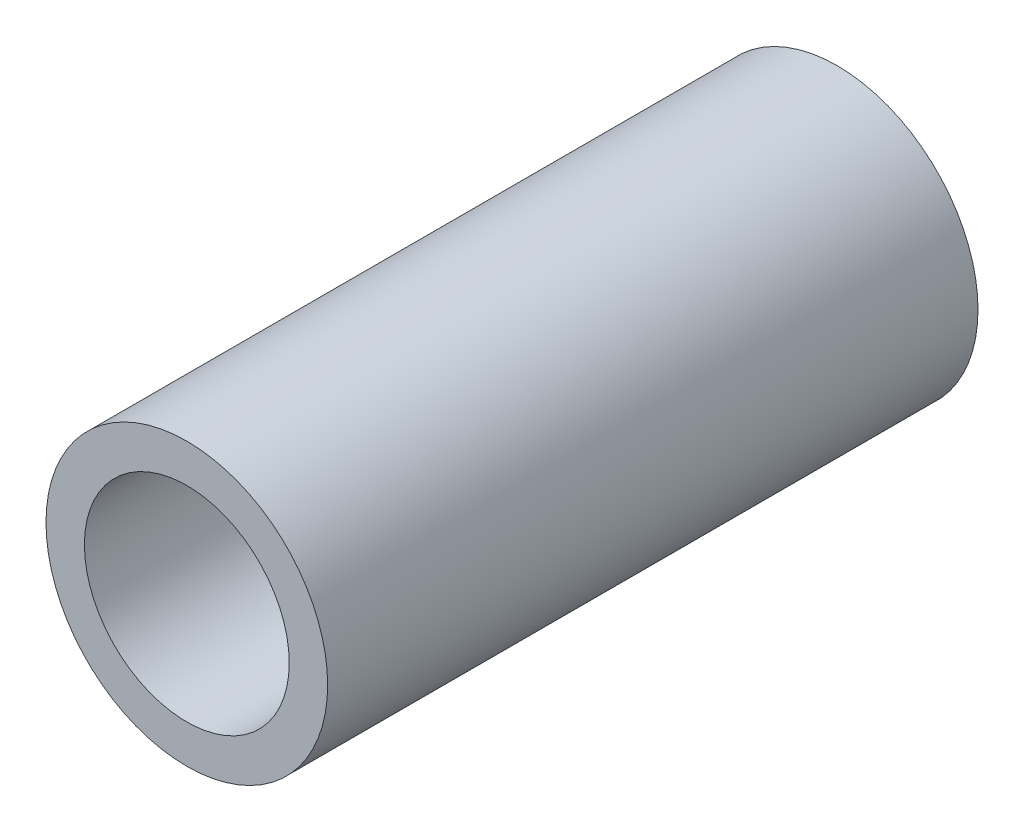
from build123d import *

# Parameters (mm, degrees)
SKETCH1_R      = 11
SKETCH1_R_2    = 8
EXTRUDE1_DEPTH = 50.8


with BuildPart() as part:
    # Sketch1 → Extrude1 (new body)
    with BuildSketch(Plane.XY):
        Circle(SKETCH1_R)
        Circle(SKETCH1_R_2, mode=Mode.SUBTRACT)
    extrude(amount=EXTRUDE1_DEPTH)


solid = part.part
